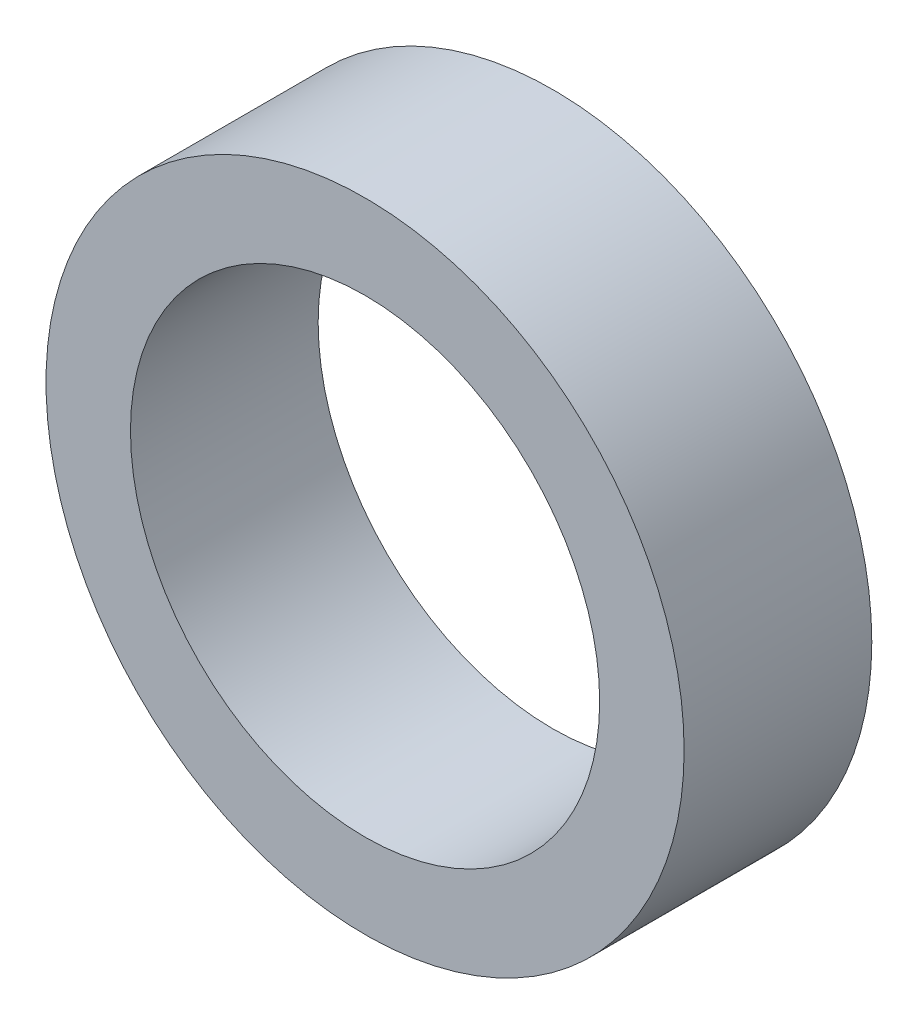
from build123d import *

# Parameters (mm, degrees)
SKETCH_1_R      = 8.5
SKETCH_1_R_2    = 6.25
EXTRUDE_1_DEPTH = 5


with BuildPart() as part:
    # 草图1 → 凸台-拉伸1 (new body)
    with BuildSketch(Plane.XY):
        Circle(SKETCH_1_R)
        Circle(SKETCH_1_R_2, mode=Mode.SUBTRACT)
    extrude(amount=EXTRUDE_1_DEPTH)


solid = part.part
